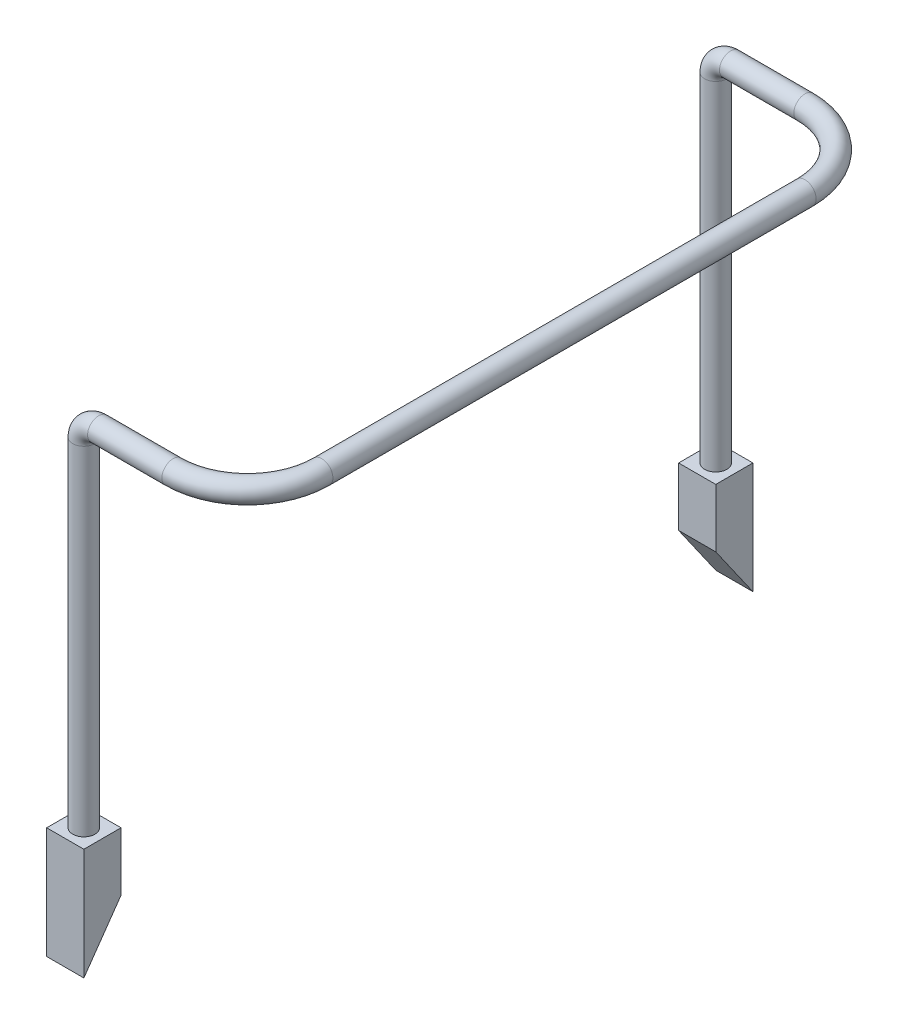
SolidWorks part; units mm, degrees
ref_plane "Front Plane" through (0, 0, 0) normal (0, 0, 1) x (1, 0, 0)
ref_plane "Top Plane" through (0, 0, 0) normal (0, 1, 0) x (1, 0, 0)
ref_plane "Right Plane" through (0, 0, 0) normal (1, 0, 0) x (0, 0, -1)
other "Configuration Table"
sketch3d "3DSketch2"
  line L0 (0, 0, 0) -> (0, 12.1, 0)
  line L1 (0.4, 12.5, 0) -> (2.4, 12.5, 0)
  line L2 (4.4, 12.5, -2) -> (4.4, 12.5, -15)
  line L3 (2.4, 12.5, -17) -> (0.4, 12.5, -17)
  line L4 (0, 12.1, -17) -> (0, 0, -17)
  arc A0 (0.4, 12.5, -17) -> (0, 12.1, -17) centre (0.4, 12.1, -17) ccw
  arc A1 (0, 12.1, 0) -> (0.4, 12.5, 0) centre (0.4, 12.1, 0) ccw
  arc A2 (4.4, 12.5, -15) -> (2.4, 12.5, -17) centre (2.4, 12.5, -15) ccw
  arc A3 (2.4, 12.5, 0) -> (4.4, 12.5, -2) centre (2.4, 12.5, -2) ccw
  point P9 (0, 12.5, -17)
  point P10 (0.4, 12.1, -16.6)
  point P13 (0, 12.5, 0)
  point P14 (0.4, 12.1, -0.4)
  point P17 (4.4, 12.5, -17)
  point P18 (2.4, 14.5, -15)
  point P21 (4.4, 12.5, 0)
  point P22 (2.4, 14.5, -2)
  dimension "D6" = 0.4
  dimension "D7" = 2
  dimension "D1" = 17
  dimension "D2" = 12.5
  dimension "D3" = 12.5
  dimension "D4" = 4.4
  dimension "D5" = 4.4
sketch "Sketch2" plane through (0, 0, 0) normal (0, 1, 0) x (1, 0, 0)
  circle A0 centre (0, 0) radius 0.3
  dimension "D1" = 0.6
sweep "Sweep1" add profiles "Sketch2" path "3DSketch2"
sketch "Sketch4" plane through (0, 0, 0) normal (0, -1, 0) x (-1, 0, 0)
  line L1 (-0.5, 16.5) -> (0.5, 16.5)
  line L2 (-0.5, 16.5) -> (-0.5, 17.5)
  line L3 (-0.5, 17.5) -> (0.5, 17.5)
  line L4 (0.5, 16.5) -> (0.5, 17.5)
  line L5 (-0.5, 16.5) -> (0.5, 17.5) construction
  line L6 (-0.5, 17.5) -> (0.5, 16.5) construction
  line L7 (-0.5, -0.5) -> (0.5, -0.5)
  line L8 (-0.5, -0.5) -> (-0.5, 0.5)
  line L9 (-0.5, 0.5) -> (0.5, 0.5)
  line L10 (0.5, -0.5) -> (0.5, 0.5)
  line L11 (-0.5, -0.5) -> (0.5, 0.5) construction
  line L12 (-0.5, 0.5) -> (0.5, -0.5) construction
  point P0 (0, 17)
  point P10 (0, 0)
  dimension "D1" = 1
  dimension "D2" = 1
  dimension "D3" = 1
  dimension "D4" = 1
extrude "Boss-Extrude1" add sketch "Sketch4" against normal blind 3
sketch "Sketch5" plane through (0, 0, 0) normal (1, 0, 0) x (0, 0, -1)
  line L0 (-0.5, 0) -> (1.5633, 2.9466)
  line L1 (1.5633, 2.9466) -> (15.4367, 2.9466)
  line L2 (15.4367, 2.9466) -> (17.5, 0)
  line L3 (17.5, 0) -> (-0.5, 0)
  line L4 (8.5, 0) -> (8.5, 5.9531) construction
  dimension "D1" = 35
  dimension "D2" = 35
extrude "Cut-Extrude1" cut sketch "Sketch5" against normal through all both and the other way through all
